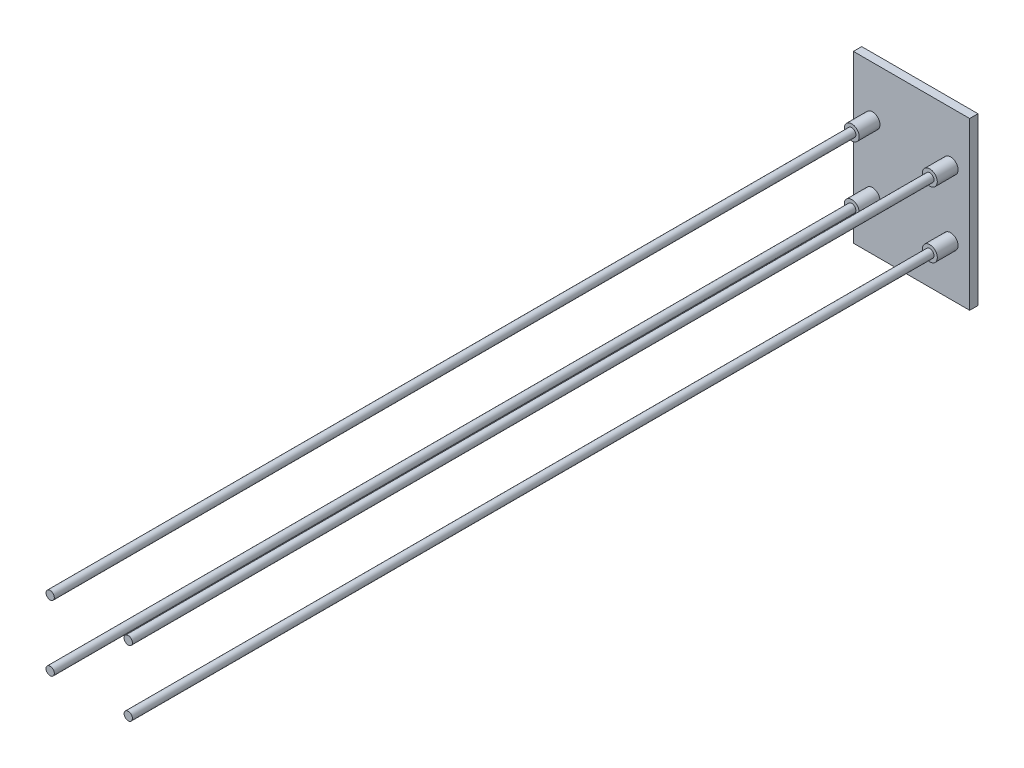
SolidWorks part; units mm, degrees
ref_plane "Front Plane" through (0, 0, 0) normal (0, 0, 1) x (1, 0, 0)
ref_plane "Top Plane" through (0, 0, 0) normal (0, 1, 0) x (1, 0, 0)
ref_plane "Right Plane" through (0, 0, 0) normal (1, 0, 0) x (0, 0, -1)
sketch "Sketch2" plane through (0, 0, 0) normal (0, 0, 1) x (1, 0, 0)
  line L1 (-59, 51.5) -> (59, 51.5) construction
  line L2 (-59, 51.5) -> (-59, -51.5) construction
  line L3 (-59, -51.5) -> (59, -51.5) construction
  line L4 (59, 51.5) -> (59, -51.5) construction
  line L5 (-59, 51.5) -> (59, -51.5) construction
  line L6 (-59, -51.5) -> (59, 51.5) construction
  line L7 (-70, 100) -> (70, 100)
  line L8 (-70, 100) -> (-70, -100)
  line L9 (-70, -100) -> (70, -100)
  line L10 (70, 100) -> (70, -100)
  line L11 (-70, 100) -> (70, -100) construction
  line L12 (-70, -100) -> (70, 100) construction
  circle A0 centre (-47, 39.5) radius 5
  circle A1 centre (-47, -39.5) radius 5
  circle A2 centre (47, 39.5) radius 5
  circle A3 centre (47, -39.5) radius 5
  point P0 (0, 0)
  point P14 (0, 0)
  dimension "D1" = 10
  dimension "D4" = 12
  dimension "D5" = 12
  dimension "D6" = 10
  dimension "D7" = 12
  dimension "D8" = 12
  dimension "D9" = 10
  dimension "D11" = 12
  dimension "D12" = 10
  dimension "D13" = 12
  dimension "D14" = 12
  dimension "D2" = 103
  dimension "D3" = 118
  dimension "D10" = 12
  dimension "D15" = 140
  dimension "D16" = 200
extrude "Boss-Extrude1" add sketch "Sketch2" along normal blind 10
sketch "Sketch3" plane through (0, 0, 10) normal (0, 0, 1) x (1, 0, 0)
  circle A0 centre (-47, 39.5) radius 9
  circle A1 centre (47, 39.5) radius 9
  circle A2 centre (-47, 39.5) radius 5
  circle A3 centre (47, 39.5) radius 5
  circle A4 centre (47, -39.5) radius 5
  circle A5 centre (47, -39.5) radius 9
  circle A6 centre (-47, -39.5) radius 5
  circle A7 centre (-47, -39.5) radius 9
  dimension "D1" = 18
  dimension "D2" = 18
  dimension "D3" = 18
  dimension "D4" = 18
extrude "Boss-Extrude2" add sketch "Sketch3" along normal blind 25
sketch "Sketch4" plane through (0, 0, 0) normal (0, 0, -1) x (-1, 0, 0)
  circle A0 centre (-47, 39.5) radius 5
  circle A1 centre (47, 39.5) radius 5
  circle A2 centre (47, -39.5) radius 5
  circle A3 centre (-47, -39.5) radius 5
extrude "Boss-Extrude3" add sketch "Sketch4" against normal blind 1000
